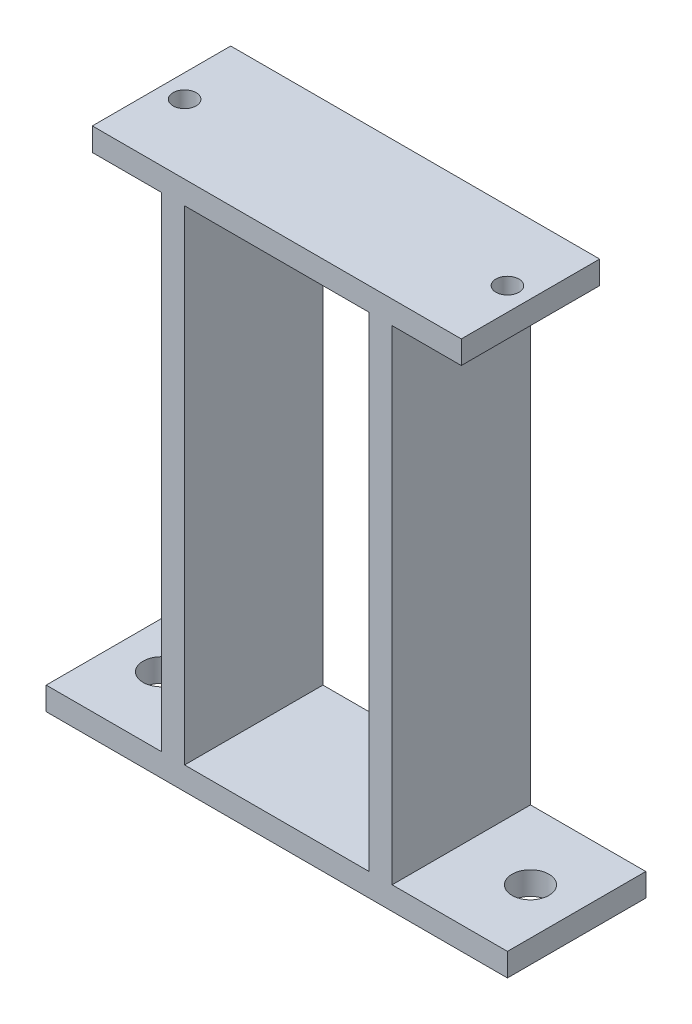
from build123d import *

# Parameters (mm, degrees)
SKETCH1_W           = 40
SKETCH1_H           = 105
BOSS_EXTRUDE1_DEPTH = 30
SKETCH2_R           = 4
CUT_EXTRUDE1_DEPTH  = 152.657508881
SKETCH3_R           = 2.5
CUT_EXTRUDE2_DEPTH  = 10


with BuildPart() as part:
    # Sketch1 → Boss-Extrude1 (new body)
    with BuildSketch(Plane.XY):
        Polygon((0, 0), (100, 0), (100, 5), (75, 5), (75, 110), (90, 110), (90, 115), (10, 115), (10, 110), (25, 110), (25, 5), (0, 5), align=None)
        with Locations((50, 57.5)):
            Rectangle(SKETCH1_W, SKETCH1_H, mode=Mode.SUBTRACT)
    extrude(amount=BOSS_EXTRUDE1_DEPTH)

    # Sketch2 → Cut-Extrude1 (cut, through all)
    with BuildSketch(Plane(origin=(0, 5, 0), x_dir=(1, 0, 0), z_dir=(0, 1, 0))):
        with Locations(Location((90, -15, 0), (0, 0, 180))):
            Circle(SKETCH2_R)
        with Locations(Location((10, -15, 0), (0, 0, 180))):
            Circle(SKETCH2_R)
    extrude(amount=-CUT_EXTRUDE1_DEPTH, mode=Mode.SUBTRACT)

    # Sketch3 → Cut-Extrude2 (cut)
    with BuildSketch(Plane(origin=(0, 115, 0), x_dir=(1, 0, 0), z_dir=(0, 1, 0))):
        with Locations(Location((15, -15, 0), (0, 0, 270))):
            Circle(SKETCH3_R)
        with Locations(Location((85, -15, 0), (0, 0, 270))):
            Circle(SKETCH3_R)
    extrude(amount=-CUT_EXTRUDE2_DEPTH, mode=Mode.SUBTRACT)


solid = part.part
